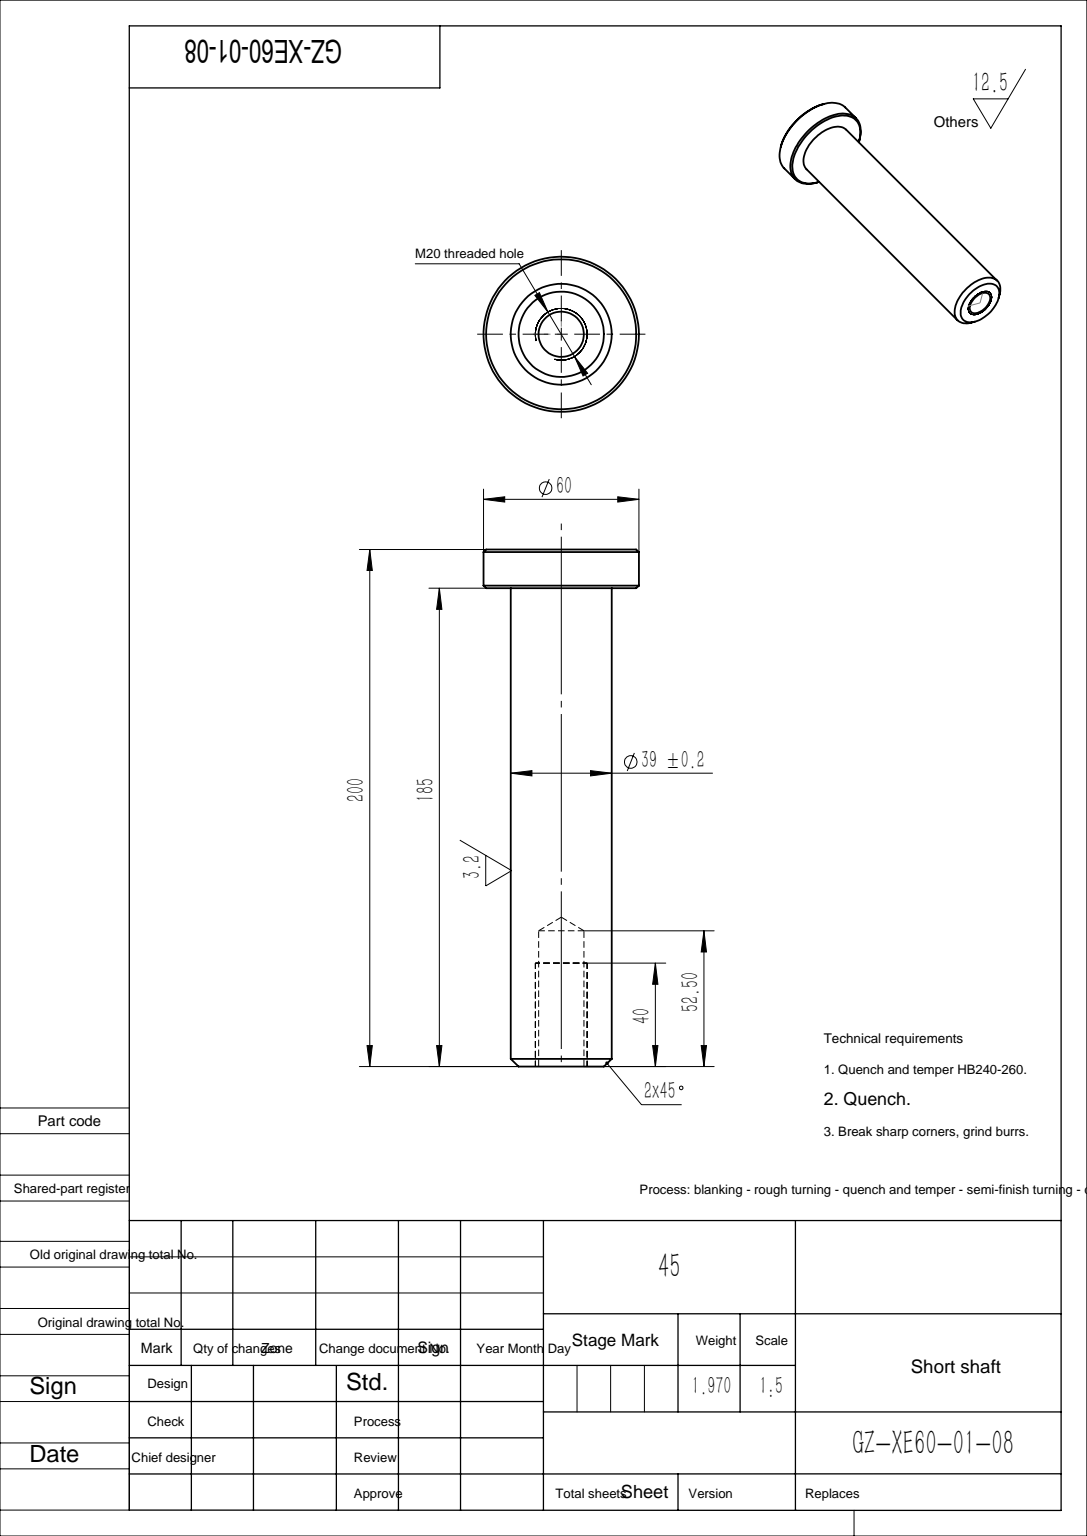
from build123d import *

# Parameters (mm, degrees)
SKETCH1_R              = 19.5
BOSS_EXTRUDE1_DEPTH    = 185
SKETCH2_R              = 30
BOSS_EXTRUDE2_DEPTH    = 15
CHAMFER1_SIZE          = 3
CHAMFER2_SIZE          = 1
M20_TAPPED_HOLE1_D     = 17.5
M20_TAPPED_HOLE1_DEPTH = 52.5
M20_TAPPED_HOLE1_TIP   = 5.257530416


with BuildPart() as part:
    # Sketch1 → Boss-Extrude1 (new body)
    with BuildSketch(Plane.XY):
        Circle(SKETCH1_R)
    extrude(amount=BOSS_EXTRUDE1_DEPTH)

    # Sketch2 → Boss-Extrude2 (add)
    with BuildSketch(Plane.XY.offset(185)):
        Circle(SKETCH2_R)
    extrude(amount=BOSS_EXTRUDE2_DEPTH)

    # Chamfer1
    chamfer1_edges = [part.edges().sort_by_distance(p)[0] for p in [
        (-19.5, 0, 0),
    ]]
    chamfer(chamfer1_edges, length=CHAMFER1_SIZE)

    # Chamfer2
    chamfer2_edges = [part.edges().sort_by_distance(p)[0] for p in [
        (-30, 0, 185),
        (-30, 0, 200),
    ]]
    chamfer(chamfer2_edges, length=CHAMFER2_SIZE)

    # M20 Tapped Hole1
    with Locations(Plane(origin=(0, 0, 0), x_dir=(-1, 0, 0), z_dir=(0, 0, -1))):
        with Locations((0, 0)):
            Hole(M20_TAPPED_HOLE1_D / 2, depth=M20_TAPPED_HOLE1_DEPTH)
            with Locations((0, 0, -(M20_TAPPED_HOLE1_DEPTH + M20_TAPPED_HOLE1_TIP / 2))):  # 118° drill point
                Cone(0, M20_TAPPED_HOLE1_D / 2, M20_TAPPED_HOLE1_TIP, mode=Mode.SUBTRACT)


solid = part.part
